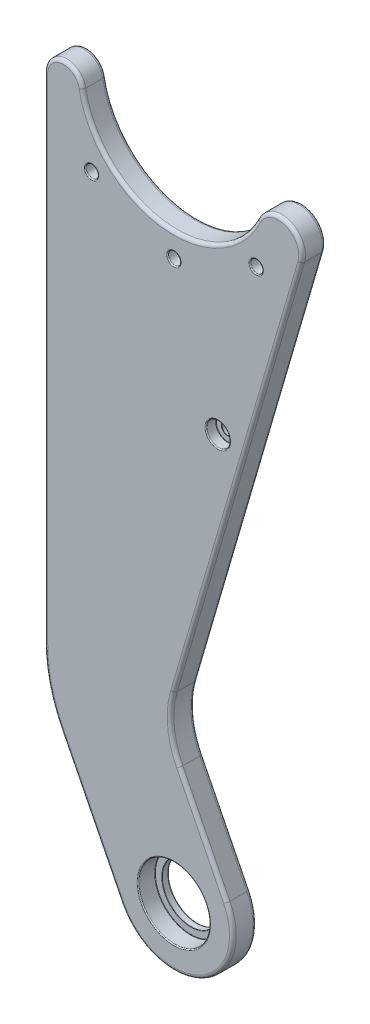
from build123d import *

# Parameters (mm, degrees)
SKETCH1_R           = 1.85
SKETCH1_R_2         = 8.5
BOSS_EXTRUDE1_DEPTH = 7
SKETCH2_R           = 10.575
CUT_EXTRUDE1_DEPTH  = 5
FILLET1_R           = 25
FILLET2_R           = 45
CUT_EXTRUDE2_REACH  = 222.975
SKETCH3_R           = 1.85
SKETCH8_R           = 3.5
CUT_EXTRUDE7_DEPTH  = 3
SKETCH9_R           = 3.5
CUT_EXTRUDE8_DEPTH  = 3
FILLET3_R           = 1
FILLET4_R           = 0.3
FILLET5_R           = 0.1


with BuildPart() as part:
    # Sketch1 → Boss-Extrude1 (new body)
    with BuildSketch(Plane.XY):
        with BuildLine():
            Line((-38.404069543, -5.740386291), (-38.404069543, -162.468720195))
            Line((-38.404069543, -162.468720195), (-15.642417773, -207.846321828))
            ThreePointArc((-15.642417773, -207.846321828), (7.846321828, -215.642417773), (15.642417773, -192.153678172))
            Line((15.642417773, -192.153678172), (-2.725328205, -155.535761851))
            Line((-2.725328205, -155.535761851), (37.73757713, -17.066323725))
            ThreePointArc((37.73757713, -17.066323725), (33.541430495, -8.573364688), (24.724946368, -12.038564163))
            ThreePointArc((24.724946368, -12.038564163), (-3.828539726, -27.232192045), (-27.085868755, -4.754546644))
            ThreePointArc((-27.085868755, -4.754546644), (-33.1968209, -0.059859271), (-38.404069543, -5.740386291))
        make_face()
        with Locations((0, -34.5)):
            Circle(SKETCH1_R, mode=Mode.SUBTRACT)
        with Locations((24.395183951, -24.395183951)):
            Circle(SKETCH1_R, mode=Mode.SUBTRACT)
        with Locations((-24.395183951, -24.395183951)):
            Circle(SKETCH1_R, mode=Mode.SUBTRACT)
        with Locations((0, -200)):
            Circle(SKETCH1_R_2, mode=Mode.SUBTRACT)
    extrude(amount=BOSS_EXTRUDE1_DEPTH)

    # Sketch2 → Cut-Extrude1 (cut)
    with BuildSketch(Plane.XY.offset(7)):
        with Locations((0, -200)):
            Circle(SKETCH2_R)
    extrude(amount=-CUT_EXTRUDE1_DEPTH, mode=Mode.SUBTRACT)

    # Fillet1
    fillet1_edges = [part.edges().sort_by_distance(p)[0] for p in [
        (-2.725328205, -155.535761851, 3.5),
    ]]
    fillet(fillet1_edges, radius=FILLET1_R)

    # Fillet2
    fillet2_edges = [part.edges().sort_by_distance(p)[0] for p in [
        (-38.404069543, -162.468720195, 3.5),
    ]]
    fillet(fillet2_edges, radius=FILLET2_R)

    # Sketch3 → Cut-Extrude2 (cut, up to next)
    with BuildSketch(Plane.XY.offset(7), mode=Mode.PRIVATE) as cut_extrude2_sk1:
        with Locations((13.025336819, -73.112909397)):
            Circle(SKETCH3_R)
    cut_extrude2_tool1 = extrude(cut_extrude2_sk1.sketch, amount=-CUT_EXTRUDE2_REACH, mode=Mode.PRIVATE) & part.part
    add(cut_extrude2_tool1.solids().sort_by_distance((13.025337, -73.112909, 7))[0], mode=Mode.SUBTRACT)

    # Sketch8 → Cut-Extrude7 (cut)
    with BuildSketch(Plane(origin=(0, 0, 0), x_dir=(-1, 0, 0), z_dir=(0, 0, -1))):
        with Locations((0, -34.5)):
            Circle(SKETCH8_R)
        with Locations((-24.395183951, -24.395183951)):
            Circle(SKETCH8_R)
        with Locations((24.395183951, -24.395183951)):
            Circle(SKETCH8_R)
    extrude(amount=-CUT_EXTRUDE7_DEPTH, mode=Mode.SUBTRACT)

    # Sketch9 → Cut-Extrude8 (cut)
    with BuildSketch(Plane.XY.offset(7)):
        with Locations((13.025336819, -73.112909397)):
            Circle(SKETCH9_R)
    extrude(amount=-CUT_EXTRUDE8_DEPTH, mode=Mode.SUBTRACT)

    # Fillet3
    fillet3_edges = [part.edges().sort_by_distance(p)[0] for p in [
        (7.846321828, -215.642417773, 0),
        (-38.404069543, -78.777777075, 0),
        (-33.1968209, -0.059859271, 0),
        (-3.828539726, -27.232192045, 0),
        (33.541430495, -8.573364688, 0),
        (18.884648871, -81.583549106, 0),
        (18.884648871, -81.583549106, 7),
        (33.541430495, -8.573364688, 7),
        (-3.828539726, -27.232192045, 7),
        (-33.1968209, -0.059859271, 7),
        (8.662142301, -178.237809376, 0),
        (8.662142301, -178.237809376, 7),
        (-0.869929821, -155.367733163, 0),
        (-38.404069543, -78.777777075, 7),
        (-0.869929821, -155.367733163, 7),
        (-24.634923651, -189.918872908, 0),
        (-24.634923651, -189.918872908, 7),
        (-37.19362994, -162.182153935, 0),
        (-37.19362994, -162.182153935, 7),
        (7.846321828, -215.642417773, 7),
    ]]
    fillet(fillet3_edges, radius=FILLET3_R)

    # Fillet4
    fillet4_edges = [part.edges().sort_by_distance(p)[0] for p in [
        (-26.245183951, -24.395183951, 7),
        (22.545183951, -24.395183951, 7),
        (-8.5, -200, 0),
        (-1.85, -34.5, 7),
        (-10.575, -200, 7),
        (11.175336819, -73.112909397, 0),
        (3.5, -34.5, 0),
        (27.895183951, -24.395183951, 0),
        (-20.895183951, -24.395183951, 0),
        (9.525336819, -73.112909397, 7),
    ]]
    fillet(fillet4_edges, radius=FILLET4_R)

    # Fillet5
    fillet5_edges = [part.edges().sort_by_distance(p)[0] for p in [
        (-10.575, -200, 2),
        (-8.5, -200, 2),
        (3.5, -34.5, 3),
        (-1.85, -34.5, 3),
        (27.895183951, -24.395183951, 3),
        (22.545183951, -24.395183951, 3),
        (-20.895183951, -24.395183951, 3),
        (-26.245183951, -24.395183951, 3),
        (9.525336819, -73.112909397, 4),
        (11.175336819, -73.112909397, 4),
    ]]
    fillet(fillet5_edges, radius=FILLET5_R)


solid = part.part
